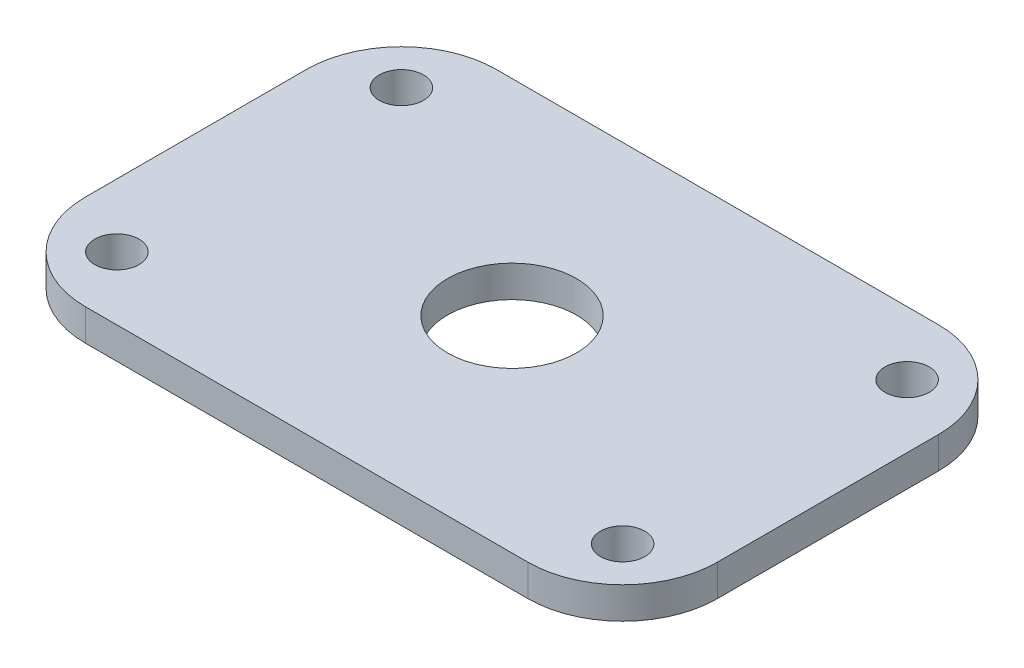
SolidWorks part; units mm, degrees
ref_plane "Front Plane" through (0, 0, 0) normal (0, 0, 1) x (1, 0, 0)
ref_plane "Top Plane" through (0, 0, 0) normal (0, 1, 0) x (1, 0, 0)
ref_plane "Right Plane" through (0, 0, 0) normal (1, 0, 0) x (0, 0, -1)
sketch "Sketch1" plane through (0, 0, 0) normal (0, 1, 0) x (1, 0, 0)
  line L1 (-35, 32.5) -> (35, 32.5)
  line L2 (-50, 17.5) -> (-50, -17.5)
  line L3 (-35, -32.5) -> (35, -32.5)
  line L4 (50, 17.5) -> (50, -17.5)
  line L5 (-50, 32.5) -> (50, -32.5) construction
  line L6 (-50, -32.5) -> (50, 32.5) construction
  arc A0 (35, 32.5) -> (50, 17.5) centre (35, 17.5) cw
  arc A1 (-50, -17.5) -> (-35, -32.5) centre (-35, -17.5) ccw
  arc A2 (-35, 32.5) -> (-50, 17.5) centre (-35, 17.5) ccw
  arc A3 (35, -32.5) -> (50, -17.5) centre (35, -17.5) ccw
  point P0 (0, 0)
  dimension "D3" = 15
  dimension "D1" = 65
  dimension "D2" = 100
extrude "Boss-Extrude1" add sketch "Sketch1" along normal blind 5
hole_wizard "M24 Tapped Hole2" positions "3DSketch2" profile "Sketch4" tap size "M24" standard "GB" end condition through all
sketch3d "3DSketch2"
  point P0 (0, 0, 0)
  point P3 (0, 5, 0)
sketch "Sketch4" plane through (0, 5, 0) normal (1, 0, 0) x (0, 0, 1)
  line L0 (0, 0) -> (0, 5)
  line L1 (0, 5) -> (10.2, 5)
  line L2 (10.2, 5) -> (10.2, 0)
  line L5 (10.2, 0) -> (0, 0)
  line L11 (0, -6.35) -> (0, 107.95) construction
  dimension "通孔螺纹孔钻头直径" = 20.4
  dimension "通孔螺纹孔钻头深度" = 5
cosmetic thread "Cosmetic thread 6" parameters "D2"=24
cosmetic thread "Cosmetic thread 7" parameters "D2"=24
hole_wizard "Hole1" positions "3DSketch3" profile "Sketch5" legacy end condition through all
sketch3d "3DSketch3"
  point P0 (-40, 5, -22.5)
  dimension "D1" = 40
  dimension "D2" = 22.5
sketch "Sketch5" plane through (-40, 5, -22.5) normal (1, 0, 0) x (0, 0, 1)
  line L0 (0, 0) -> (0, 5)
  line L1 (0, 5) -> (3.5, 5)
  line L2 (3.5, 5) -> (3.5, 0)
  line L3 (3.5, 0) -> (0, 0)
  line L4 (0, 110) -> (0, -10) construction
  dimension "直径" = 7
  dimension "深度" = 5
pattern_linear "LPattern1" count 2 spacing 80 along (1, 0, 0) count 2 spacing 45 along (0, 0, 1) of "Hole1"
